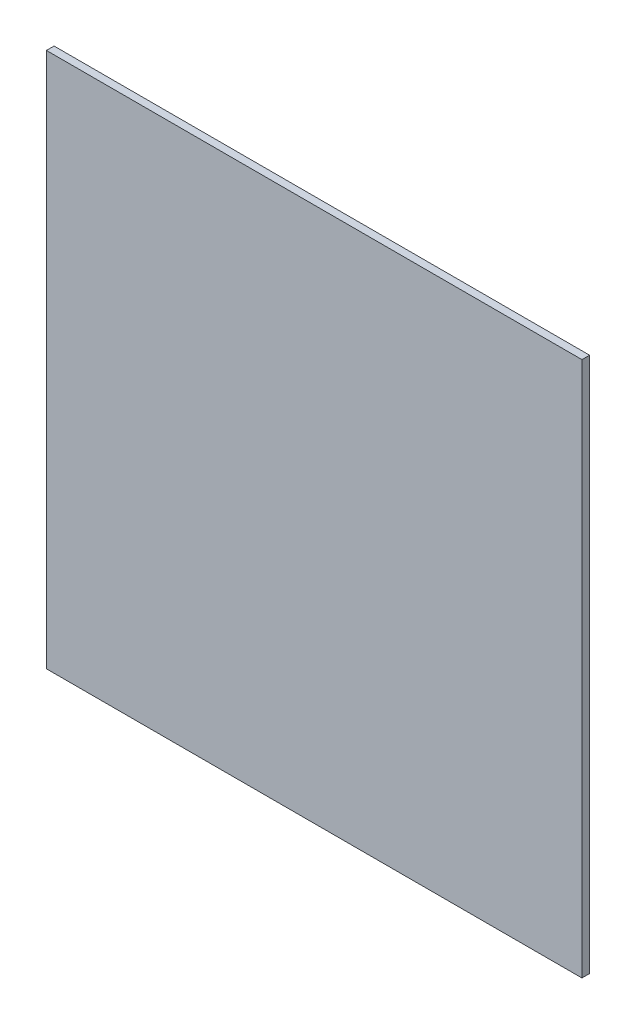
from build123d import *

# Parameters (mm, degrees)
SKETCH_1_W      = 280
SKETCH_1_H      = 280
EXTRUDE_1_DEPTH = 2


with BuildPart() as part:
    # 草图1 → 凸台-拉伸1 (new, symmetric)
    with BuildSketch(Plane.XY):
        Rectangle(SKETCH_1_W, SKETCH_1_H)
    extrude(amount=EXTRUDE_1_DEPTH, both=True)


solid = part.part
